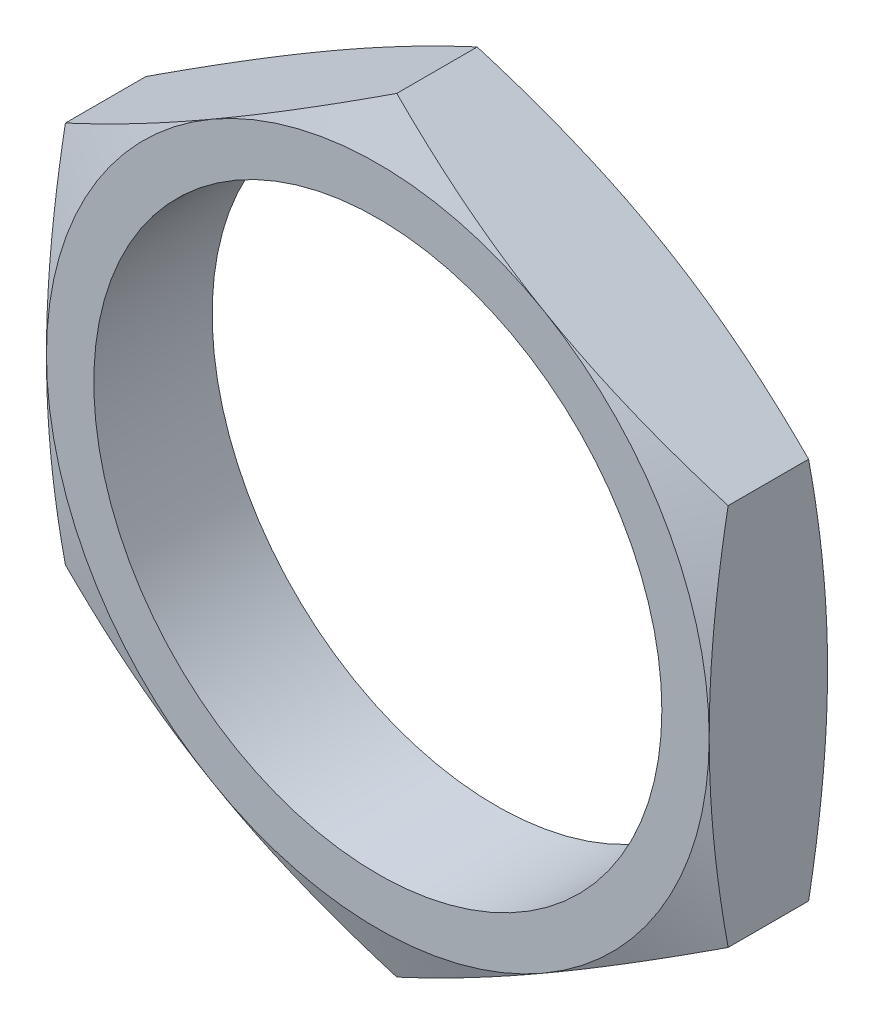
SolidWorks part; units mm, degrees
ref_plane "Front Plane" through (0, 0, 0) normal (0, 0, 1) x (1, 0, 0)
ref_plane "Top Plane" through (0, 0, 0) normal (0, 1, 0) x (1, 0, 0)
ref_plane "Right Plane" through (0, 0, 0) normal (1, 0, 0) x (0, 0, -1)
sketch "Sketch1" plane through (0, 0, 0) normal (0, 0, 1) x (1, 0, 0)
  line L1 (0, 8.0829) -> (-7, 4.0415)
  line L2 (-7, 4.0415) -> (-7, -4.0415)
  line L3 (-7, -4.0415) -> (0, -8.0829)
  line L4 (0, -8.0829) -> (7, -4.0415)
  line L5 (7, -4.0415) -> (7, 4.0415)
  line L6 (7, 4.0415) -> (0, 8.0829)
  circle A0 centre (0, 0) radius 7 construction
  circle A1 centre (0, 0) radius 6
  dimension "D1" = 14
  dimension "D2" = 12
extrude "Boss-Extrude1" add sketch "Sketch1" along normal blind 2.5
cosmetic thread "Cosmetic Thread1" parameters "D2"=12.0001
sketch "Sketch3" plane through (0, 0, 0) normal (1, 0, 0) x (0, 0, -1)
  line L0 (-2.5, 8.0829) -> (-2.1, 8.0829)
  line L1 (-2.5, 8.0829) -> (0, 8.0829) construction
  line L2 (0, 0) -> (-2.5, 0) construction
  line L3 (-2.5, 7) -> (-2.5, 8.0829)
  line L4 (0, 8.0829) -> (-0.4, 8.0829)
  line L5 (-2.5, 7) -> (-2.1, 8.0829)
  line L6 (-2.5, 7) -> (0, 7) construction
  line L7 (0, 8.0829) -> (0, 7)
  line L8 (0, 7) -> (-0.4, 8.0829)
  dimension "D1" = 0.4
  dimension "D2" = 0.4
  dimension "D3" = 7
revolve "Cut-Revolve1" cut sketch "Sketch3" angle 360 about L2
